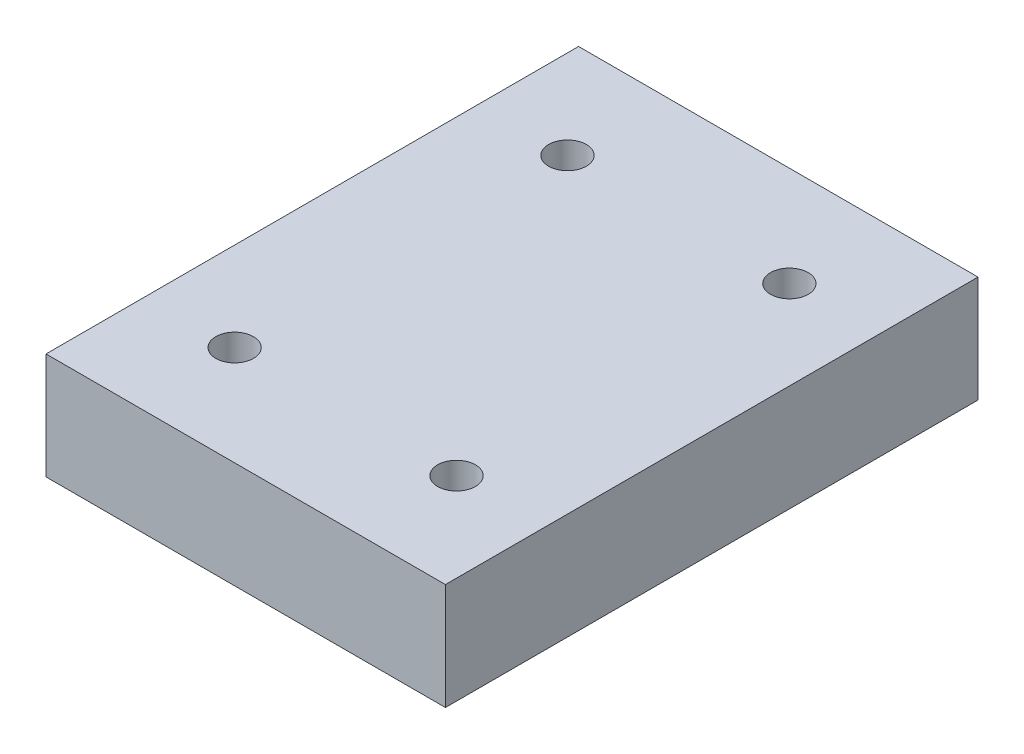
SolidWorks part; units mm, degrees
material "A3"
ref_plane "前视基准面" through (0, 0, 0) normal (0, 0, 1) x (1, 0, 0)
ref_plane "上视基准面" through (0, 0, 0) normal (0, 1, 0) x (1, 0, 0)
ref_plane "右视基准面" through (0, 0, 0) normal (1, 0, 0) x (0, 0, -1)
sketch "草图1" plane through (0, 0, 0) normal (0, 1, 0) x (1, 0, 0)
  line L1 (-45, -60) -> (45, -60)
  line L2 (-45, -60) -> (-45, 60)
  line L3 (-45, 60) -> (45, 60)
  line L4 (45, -60) -> (45, 60)
  line L5 (-45, -60) -> (45, 60) construction
  line L6 (-45, 60) -> (45, -60) construction
  point P0 (0, 0)
  dimension "D1" = 120
  dimension "D2" = 90
extrude "凸台-拉伸1" add sketch "草图1" along normal blind 24
hole_wizard "M10 螺纹孔1" positions "草图2" profile "草图3" tap size "M10" standard "GB" end condition through all
sketch "草图2" plane through (0, 24, 0) normal (0, 1, 0) x (1, 0, 0)
  line L0 (0, 60) -> (0, 0) construction
  line L1 (45, 60) -> (-45, 60) construction
  line L2 (0, 0) -> (45, 0) construction
  line L3 (45, -60) -> (45, 60) construction
  point P0 (-25, -37.5)
  point P14 (-25, 37.5)
  point P15 (25, 37.5)
  point P16 (25, -37.5)
  dimension "D1" = 50
  dimension "D2" = 75
sketch "草图3" plane through (-25, 24, 37.5) normal (1, 0, 0) x (0, 0, 1)
  line L0 (0, 0) -> (0, 24)
  line L1 (0, 24) -> (4.25, 24)
  line L2 (4.25, 24) -> (4.25, 0)
  line L5 (4.25, 0) -> (0, 0)
  line L11 (0, -6.35) -> (0, 107.95) construction
  dimension "通孔螺纹孔钻头直径" = 8.5
  dimension "通孔螺纹孔钻头深度" = 24
cosmetic thread "孔螺蚊线1"
cosmetic thread "孔螺蚊线2"
cosmetic thread "孔螺蚊线3"
cosmetic thread "孔螺蚊线4"
